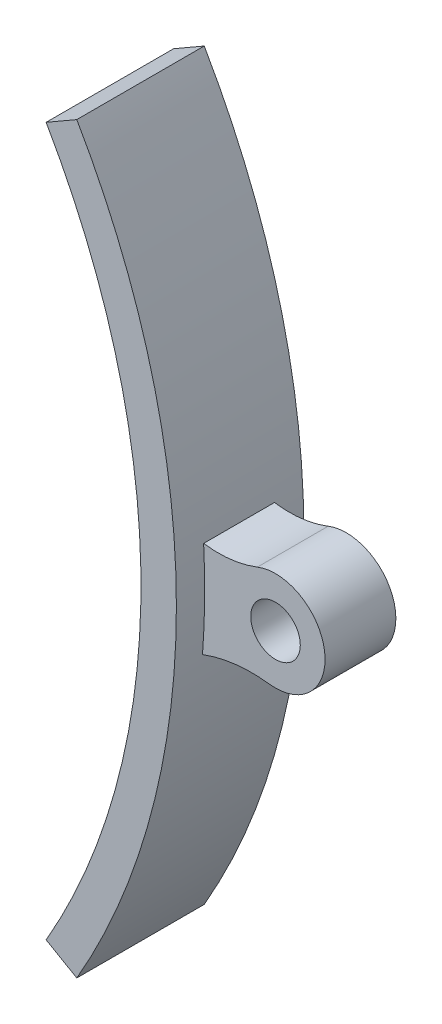
SolidWorks part; units mm, degrees
ref_plane "前视基准面" through (0, 0, 0) normal (0, 0, 1) x (1, 0, 0)
ref_plane "上视基准面" through (0, 0, 0) normal (0, 1, 0) x (1, 0, 0)
ref_plane "右视基准面" through (0, 0, 0) normal (1, 0, 0) x (0, 0, -1)
other "Configuration Table"
sketch "草图1" plane through (0, 0, 0) normal (0, 0, 1) x (1, 0, 0)
  line L0 (-191.767, 0) -> (227.8528, 0) construction
  line L1 (0, 138.01) -> (0, -143.3557) construction
  line L2 (0, 0) -> (165.9334, 95.8017) construction
  line L3 (0, 0) -> (165.9334, -95.8017) construction
  line L4 (86.6025, 50) -> (90.9327, 52.5)
  line L5 (86.6025, -50) -> (90.9327, -52.5)
  line L6 (105, 0) -> (195.6333, 0) construction
  arc A0 (90.9327, -52.5) -> (90.9327, 52.5) centre (0, 0) ccw
  arc A1 (86.6025, -50) -> (86.6025, 50) centre (0, 0) ccw
  dimension "D1" = 30
extrude "凸台-拉伸1" add sketch "草图1" along normal blind 18 contours L5 A0 L4 A1
ref_plane "基准面1" through (105, 0, 0) normal (1, 0, 0) x (0, 0, -1)
ref_plane "基准面3" through (0, 0, 9) normal (0, 0, 1) x (1, 0, 0)
sketch "草图8" plane through (0, 0, 9) normal (0, 0, 1) x (1, 0, 0)
  line L0 (115, 0) -> (121.0706, 0) construction
  line L1 (115, 0) -> (86.7653, 0) construction
  line L2 (103.4686, 5.8789) -> (102.7264, -8.9074)
  circle A0 centre (115, 0) radius 3.5
  arc A1 (114.1377, -6.9467) -> (112.4361, 6.5136) centre (115, 0) ccw
  arc A2 (103.4686, 5.8789) -> (112.4361, 6.5136) centre (106.942, 20.4712) ccw
  arc A3 (114.1377, -6.9467) -> (102.7264, -8.9074) centre (111.6739, -26.7944) ccw
  dimension "D1" = 115
extrude "凸台-拉伸5" add sketch "草图8" along normal mid plane 10
